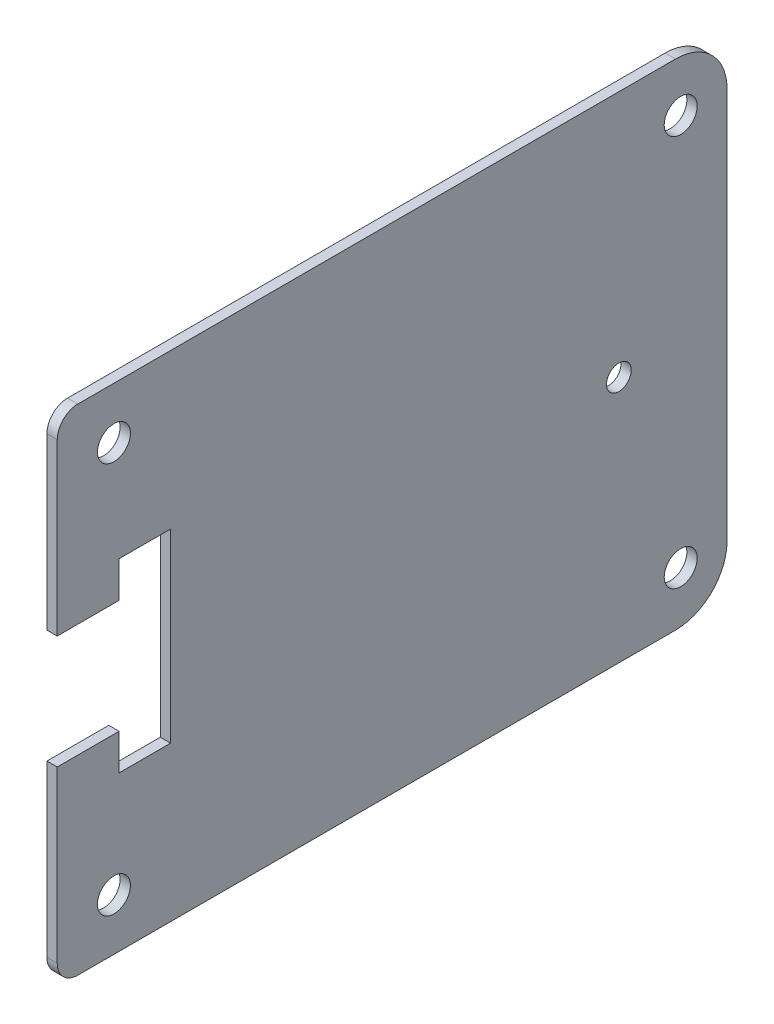
from build123d import *

# Parameters (mm, degrees)
SKETCH_1_W                = 65
SKETCH_1_H                = 48
EXTRUDE_1_DEPTH           = 20
SKETCH_2_W                = 6
SKETCH_2_H                = 27.1
CUT_EXTRUDE_1_DEPTH       = 80
CUT_EXTRUDE_2_DEPTH       = 80
SKETCH_4_R                = 1.2
CUT_EXTRUDE_3_DEPTH       = 6
HOLE_WIZARD_1_D           = 3.4
HOLE_WIZARD_1_CBORE_D     = 6
HOLE_WIZARD_1_CBORE_DEPTH = 5
FILLET_1_R                = 5
SKETCH_9_W                = 19.082133463
SKETCH_9_H                = 84.157101427
CUT_EXTRUDE_6_DEPTH       = 120
SKETCH_10_W               = 25.015989719
SKETCH_10_H               = 30.267159573
EXTRUDE_2_DEPTH           = 1
SKETCH_11_R               = 1.6
CUT_EXTRUDE_7_DEPTH       = 120
FILLET_2_R                = 2


with BuildPart() as part:
    # 草图1 → 凸台-拉伸1 (new body)
    with BuildSketch(Plane(origin=(0, 0, 0), x_dir=(0, 0, -1), z_dir=(1, 0, 0))):
        Rectangle(SKETCH_1_W, SKETCH_1_H)
    extrude(amount=EXTRUDE_1_DEPTH)

    # 草图2 → 切除-拉伸1 (cut)
    with BuildSketch(Plane(origin=(0, 0, -32.5), x_dir=(-1, 0, 0), z_dir=(0, 0, -1))):
        Rectangle(SKETCH_2_W, SKETCH_2_H)
    extrude(amount=-CUT_EXTRUDE_1_DEPTH, mode=Mode.SUBTRACT)

    # 草图3 → 切除-拉伸2 (cut)
    with BuildSketch(Plane(origin=(20, 0, 0), x_dir=(0, 0, -1), z_dir=(1, 0, 0))):
        Polygon((-26.5, -9), (-21.5, -9), (-21.5, 9), (-26.5, 9), (-26.5, 5.5), (-32.5, 5.5), (-32.5, -5.5), (-26.5, -5.5), align=None)
    extrude(amount=-CUT_EXTRUDE_2_DEPTH, mode=Mode.SUBTRACT)

    # 草图4 → 切除-拉伸3 (cut)
    with BuildSketch(Plane(origin=(20, 0, 0), x_dir=(0, 0, -1), z_dir=(1, 0, 0))):
        with Locations((22, 0)):
            Circle(SKETCH_4_R)
    extrude(amount=-CUT_EXTRUDE_3_DEPTH, mode=Mode.SUBTRACT)

    # 打孔尺寸(%根据)开槽圆柱头螺钉的类型1 (through all)
    with Locations(Plane(origin=(20, 0, 0), x_dir=(0, 0, -1), z_dir=(1, 0, 0))):
        with Locations((7.35, -10), (-7.65, -10), (-7.65, 10), (7.35, 10)):
            CounterBoreHole(HOLE_WIZARD_1_D / 2, HOLE_WIZARD_1_CBORE_D / 2, HOLE_WIZARD_1_CBORE_DEPTH)

    # 圆角1
    fillet_1_edges = [part.edges().sort_by_distance(p)[0] for p in [
        (10, -24, -32.5),
        (10, 24, -32.5),
    ]]
    fillet(fillet_1_edges, radius=FILLET_1_R)

    # 草图9 → 切除-拉伸6 (cut)
    with BuildSketch(Plane(origin=(0, 24, 0), x_dir=(1, 0, 0), z_dir=(0, 1, 0))):
        with Locations((9.458933268, -0.081547579)):
            Rectangle(SKETCH_9_W, SKETCH_9_H)
    extrude(amount=-CUT_EXTRUDE_6_DEPTH, mode=Mode.SUBTRACT)

    # 草图10 → 凸台-拉伸2 (add)
    with BuildSketch(Plane.ZY.offset(-19)):
        with Locations((0.80226206, -0.656396231)):
            Rectangle(SKETCH_10_W, SKETCH_10_H)
    extrude(amount=-EXTRUDE_2_DEPTH)

    # 草图11 → 切除-拉伸7 (cut)
    with BuildSketch(Plane.ZY.offset(-19)):
        with Locations((-28, 19)):
            Circle(SKETCH_11_R)
        with Locations((-28, -19)):
            Circle(SKETCH_11_R)
        with Locations((27, -19)):
            Circle(SKETCH_11_R)
        with Locations(Location((27, 19, 0), (0, 0, 180))):
            Circle(SKETCH_11_R)
    extrude(amount=-CUT_EXTRUDE_7_DEPTH, mode=Mode.SUBTRACT)

    # 圆角2
    fillet_2_edges = [part.edges().sort_by_distance(p)[0] for p in [
        (19.5, -24, 32.5),
        (19.5, 24, 32.5),
    ]]
    fillet(fillet_2_edges, radius=FILLET_2_R)


solid = part.part
